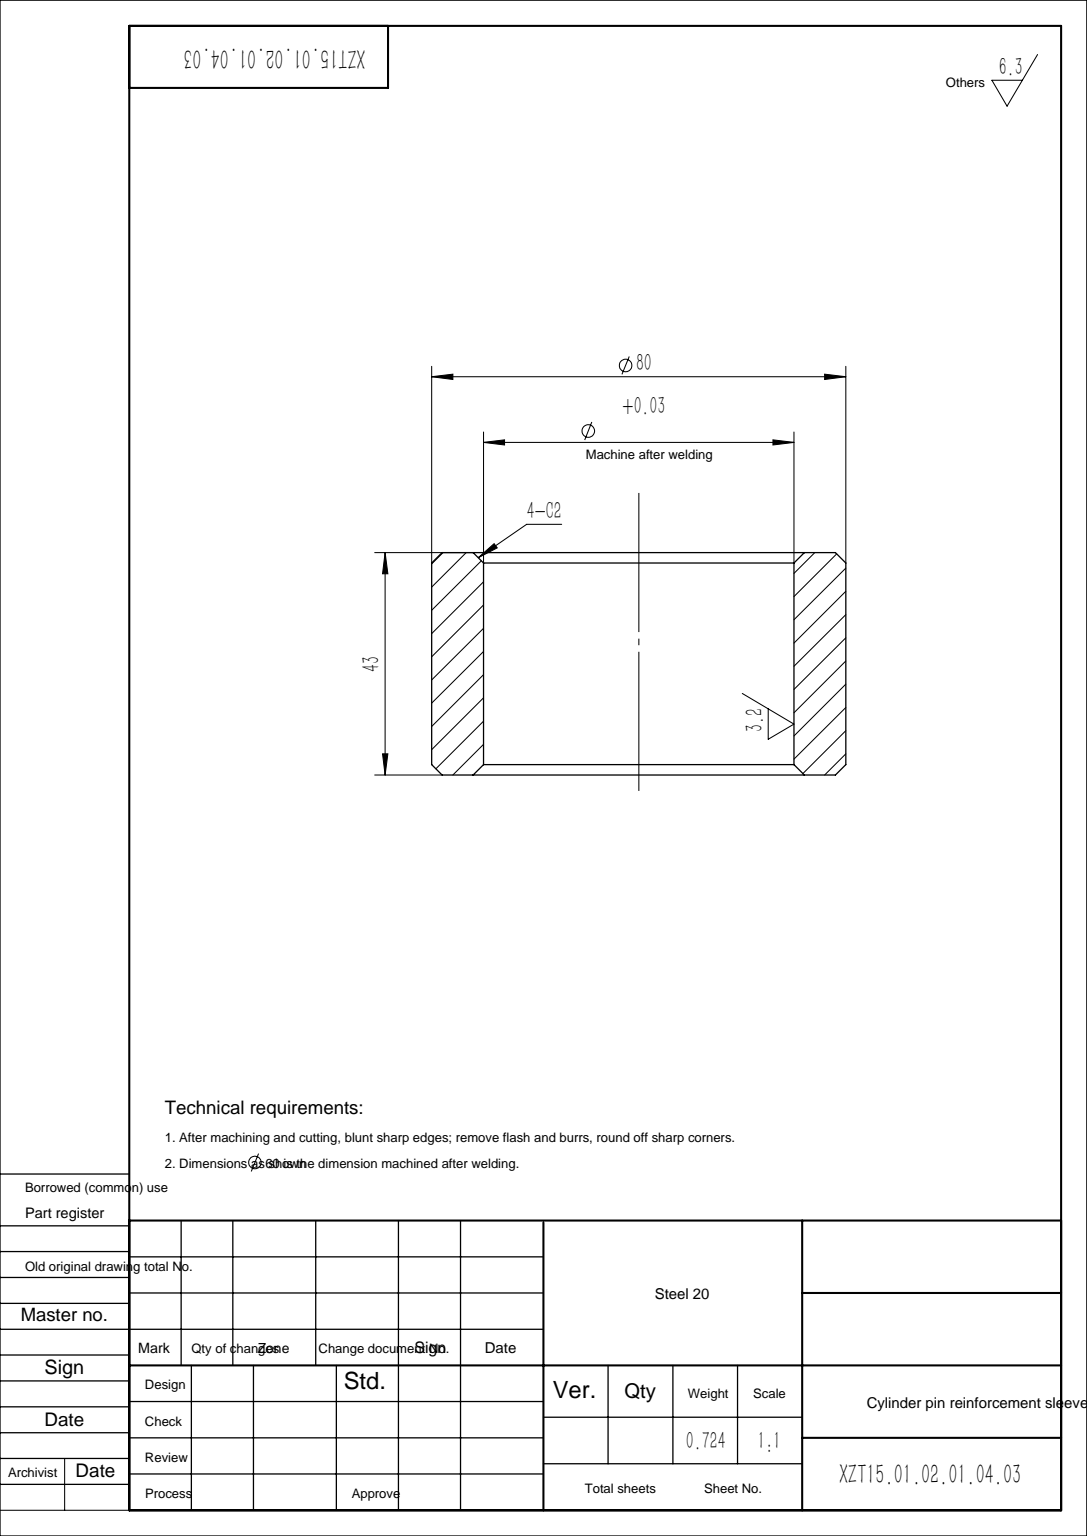
from build123d import *

# Parameters (mm, degrees)
SKETCH1_R           = 40
SKETCH1_R_2         = 30
BOSS_EXTRUDE1_DEPTH = 43
CHAMFER2_SIZE       = 2


with BuildPart() as part:
    # Sketch1 → Boss-Extrude1 (new body)
    with BuildSketch(Plane(origin=(0, 0, 0), x_dir=(1, 0, 0), z_dir=(0, 1, 0))):
        with Locations(Location((0, 0, 0), (0, 0, 270))):
            Circle(SKETCH1_R)
        with Locations(Location((0, 0, 0), (0, 0, 270))):
            Circle(SKETCH1_R_2, mode=Mode.SUBTRACT)
    extrude(amount=BOSS_EXTRUDE1_DEPTH)

    # Chamfer2
    chamfer2_edges = [part.edges().sort_by_distance(p)[0] for p in [
        (0, 0, -40),
        (0, 43, -40),
        (0, 0, -30),
        (0, 43, -30),
    ]]
    chamfer(chamfer2_edges, length=CHAMFER2_SIZE)


solid = part.part
